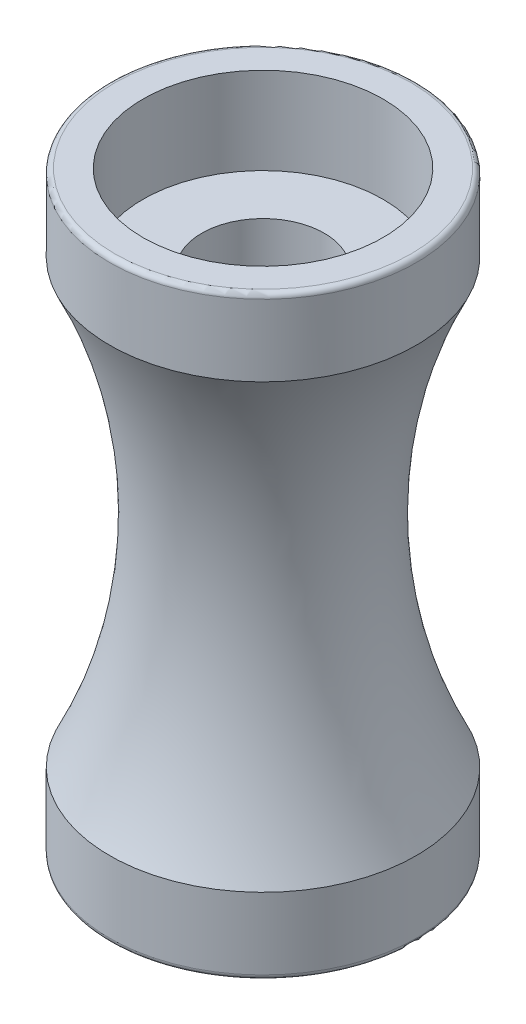
SolidWorks part; units mm, degrees
ref_plane "前视基准面" through (0, 0, 0) normal (0, 0, 1) x (1, 0, 0)
ref_plane "上视基准面" through (0, 0, 0) normal (0, 1, 0) x (1, 0, 0)
ref_plane "右视基准面" through (0, 0, 0) normal (1, 0, 0) x (0, 0, -1)
sketch "草图1" plane through (0, 0, 0) normal (0, 0, 1) x (1, 0, 0)
  line L0 (0, 0) -> (0, 116.5)
  line L1 (0, 116.5) -> (30, 116.5)
  line L2 (30, 116.5) -> (30, 101.5)
  line L3 (0, 0) -> (30, 0)
  line L4 (30, 0) -> (30, 15)
  arc A0 (30, 101.5) -> (30, 15) centre (118.5281, 58.25) ccw
  point P8 (20, 58.25)
  dimension "D1" = 116.5
  dimension "D2" = 30
  dimension "D3" = 30
  dimension "D4" = 15
  dimension "D5" = 15
  dimension "D6" = 20
revolve "旋转1" add sketch "草图1" angle 360 about L0
sketch "草图2" plane through (0, 116.5, 0) normal (0, 1, 0) x (1, 0, 0)
  circle A0 centre (0, 0) radius 12
  dimension "D1" = 24
extrude "切除-拉伸1" cut sketch "草图2" against normal up to surface (116.5 mm away) up to face at (0, 0, -30)
sketch "草图3" plane through (0, 116.5, 0) normal (0, 1, 0) x (1, 0, 0)
  circle A0 centre (0, 0) radius 23.5
  circle A1 centre (0, 0) radius 10
  dimension "D1" = 47
  dimension "D2" = 20
extrude "切除-拉伸2" cut sketch "草图3" against normal blind 17
sketch "草图4" plane through (0, 0, 0) normal (0, -1, 0) x (1, 0, 0)
  circle A0 centre (0, 0) radius 23.5
  circle A1 centre (0, 0) radius 10
  dimension "D1" = 47
  dimension "D2" = 20
extrude "切除-拉伸3" cut sketch "草图4" against normal blind 17
fillet "圆角1" radius 1 2 edges at (0, 116.5, -30) (0, 0, -30)
